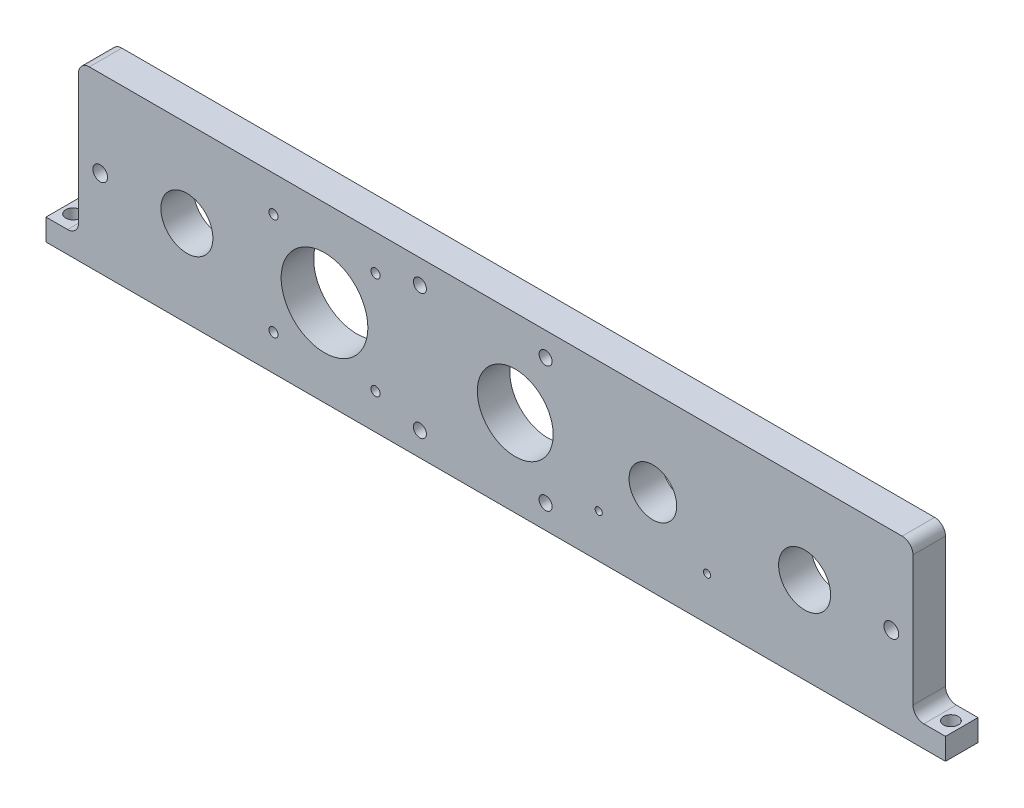
SolidWorks part; units mm, degrees
material "6061 合金"
ref_plane "Front Plane" through (0, 0, 0) normal (0, 0, 1) x (1, 0, 0)
ref_plane "Top Plane" through (0, 0, 0) normal (0, 1, 0) x (1, 0, 0)
ref_plane "Right Plane" through (0, 0, 0) normal (1, 0, 0) x (0, 0, -1)
sketch "Sketch1" plane through (0, 0, 0) normal (0, 0, 1) x (1, 0, 0)
  line L0 (0, 0) -> (0, 85.4446) construction
  line L1 (207.5, 0) -> (-207.5, 0)
  line L2 (-207.5, 0) -> (-207.5, 10)
  line L3 (-207.5, 10) -> (-192.5, 10)
  line L4 (-192.5, 10) -> (-192.5, 70)
  line L5 (-192.5, 70) -> (-207.5, 70)
  line L6 (-207.5, 70) -> (-207.5, 80)
  line L7 (-207.5, 80) -> (207.5, 80)
  line L8 (207.5, 70) -> (207.5, 80)
  line L9 (192.5, 70) -> (207.5, 70)
  line L10 (192.5, 10) -> (192.5, 70)
  line L11 (207.5, 10) -> (192.5, 10)
  line L12 (207.5, 0) -> (207.5, 10)
  point P11 (0, 80)
  dimension "D1" = 80
  dimension "D2" = 10
  dimension "D3" = 10
  dimension "D4" = 15
  dimension "D5" = 415
extrude "Boss-Extrude1" add sketch "Sketch1" along normal mid plane 15
sketch "Sketch2" plane through (0, 0, 7.5) normal (0, 0, 1) x (1, 0, 0)
  line L0 (-192.5, 40) -> (192.5, 40) construction
  line L1 (-192.5, 70) -> (-192.5, 10) construction
  line L2 (192.5, 10) -> (192.5, 70) construction
  circle A0 centre (-142.5, 40) radius 12
  circle A3 centre (9, 40) radius 17.5
  circle A4 centre (72.5, 40) radius 11
  circle A5 centre (-79, 40) radius 20
  circle A6 centre (142.5, 40) radius 12
  circle A7 centre (-182.5, 40) radius 3.4
  circle A8 centre (182.5, 40) radius 3.4
  dimension "D2" = 24
  dimension "D3" = 40
  dimension "D4" = 10
  dimension "D5" = 6.8
  dimension "D6" = 6.8
  dimension "D7" = 63.5
  dimension "D8" = 63.5
  dimension "D9" = 22
  dimension "D10" = 35
  dimension "D11" = 40
  dimension "D12" = 40
  dimension "D13" = 88
  dimension "D14" = 24
  dimension "D15" = 70
  dimension "D16" = 50
  dimension "D17" = 10
extrude "Cut-Extrude1" cut sketch "Sketch2" against normal blind 15
sketch "Sketch3" plane through (0, 0, 7.5) normal (0, 0, 1) x (1, 0, 0)
  line L0 (9, 40) -> (-6, 40) construction
  line L1 (23, 11) -> (-35, 11) construction
  line L2 (23, 11) -> (23, 69) construction
  line L3 (23, 69) -> (-35, 69) construction
  line L4 (-35, 11) -> (-35, 69) construction
  line L5 (23, 11) -> (-35, 69) construction
  line L6 (23, 69) -> (-35, 11) construction
  circle A0 centre (-35, 69) radius 3
  circle A1 centre (23, 69) radius 3
  circle A2 centre (23, 11) radius 3
  circle A3 centre (-35, 11) radius 3
  point P0 (-6, 40)
  dimension "D3" = 6
  dimension "D1" = 58
  dimension "D2" = 15
extrude "Cut-Extrude2" cut sketch "Sketch3" against normal blind 15
sketch "Sketch4" plane through (0, 80, 0) normal (0, 1, 0) x (1, 0, 0)
  line L0 (-207.5, 0) -> (0, 0) construction
  line L1 (-207.5, -7.5) -> (-207.5, 7.5) construction
  line L2 (0, 0) -> (0, 7.5) construction
  line L3 (207.5, 7.5) -> (-207.5, 7.5) construction
  circle A0 centre (-202.5, 0) radius 3.4
  circle A1 centre (202.5, 0) radius 3.4
  dimension "D1" = 6.8
  dimension "D2" = 5
extrude "Cut-Extrude3" cut sketch "Sketch4" against normal through all
fillet "Fillet1" radius 5 4 edges at (-192.5, 10, 0) (-192.5, 70, 0) (192.5, 10, 0) (192.5, 70, 0)
hole_wizard "M4 Tapped Hole1" positions "Sketch6" profile "Sketch7" tap size "M4" standard "GB" end condition through all
sketch "Sketch6" plane through (0, 0, 7.5) normal (0, 0, 1) x (1, 0, 0)
  line L0 (97.5, 20) -> (47.5, 20) construction
  line L2 (72.5, 40) -> (72.5, 20) construction
  point P0 (47.5, 20)
  point P2 (97.5, 20)
  dimension "D1" = 20
  dimension "D2" = 50
sketch "Sketch7" plane through (47.5, 20, 7.5) normal (1, 0, 0) x (0, -1, 0)
  line L0 (0, 0) -> (0, 15)
  line L1 (0, 15) -> (1.65, 15)
  line L2 (1.65, 15) -> (1.65, 0)
  line L5 (1.65, 0) -> (0, 0)
  line L11 (0, -6.35) -> (0, 107.95) construction
  dimension "通孔螺纹孔钻头直径" = 3.3
  dimension "通孔螺纹孔钻头深度" = 15
cosmetic thread "Hole Thread2" parameters "D2"=4
cosmetic thread "Hole Thread7" parameters "D2"=4
hole_wizard "M5 Tapped Hole1" positions "Sketch8" profile "Sketch9" tap size "M5" standard "GB" end condition up to next
sketch "Sketch8" plane through (0, 0, 7.5) normal (0, 0, 1) x (1, 0, 0)
  line L1 (-102.55, 63.55) -> (-55.45, 63.55) construction
  line L2 (-102.55, 63.55) -> (-102.55, 16.45) construction
  line L3 (-102.55, 16.45) -> (-55.45, 16.45) construction
  line L4 (-55.45, 63.55) -> (-55.45, 16.45) construction
  line L5 (-79, 40) -> (-79, 16.45) construction
  line L7 (-55.45, 40) -> (-79, 40) construction
  point P1 (-102.55, 63.55)
  point P2 (-55.45, 16.45)
  point P57 (-102.55, 16.45)
  point P58 (-55.45, 63.55)
  dimension "D1" = 47.1
sketch "Sketch9" plane through (-102.55, 63.55, 7.5) normal (1, 0, 0) x (0, -1, 0)
  line L0 (0, 0) -> (0, 15)
  line L1 (0, 15) -> (2.1, 15)
  line L2 (2.1, 15) -> (2.1, 0)
  line L5 (2.1, 0) -> (0, 0)
  line L11 (0, -6.35) -> (0, 107.95) construction
  dimension "通孔螺纹孔钻头直径" = 4.2
  dimension "通孔螺纹孔钻头深度" = 15
cosmetic thread "Hole Thread3" parameters "D2"=5
cosmetic thread "Hole Thread4" parameters "D2"=5
cosmetic thread "Hole Thread5" parameters "D2"=5
cosmetic thread "Hole Thread6" parameters "D2"=5
sketch "Sketch10" plane through (0, 0, 7.5) normal (0, 0, 1) x (1, 0, 0)
  line L0 (-192.5, 65) -> (-192.5, 15) construction
  line L1 (-192.5, 40) -> (-207.5, 40)
  line L2 (-192.5, 40) -> (-192.5, 80)
  line L3 (-192.5, 80) -> (-207.5, 80)
  line L4 (-207.5, 40) -> (-207.5, 80)
  line L5 (192.5, 15) -> (192.5, 65) construction
  line L6 (192.5, 40) -> (207.5, 40)
  line L7 (192.5, 40) -> (192.5, 80)
  line L8 (192.5, 80) -> (207.5, 80)
  line L9 (207.5, 40) -> (207.5, 80)
extrude "Cut-Extrude4" cut sketch "Sketch10" against normal through all
fillet "Fillet2" radius 5 2 edges at (192.5, 80, 0) (-192.5, 80, 0)
hole_wizard "M6 Tapped Hole1" positions "Sketch11" profile "Sketch12" tap size "M6" standard "GB"
sketch "Sketch11" plane through (0, 0, 0) normal (0, -1, 0) x (-1, 0, 0)
  line L0 (-207.5, 0) -> (-125, 0) construction
  line L1 (-207.5, -7.5) -> (-207.5, 7.5) construction
  line L2 (-125, 0) -> (125, 0) construction
  point P0 (-125, 0)
  point P2 (125, 0)
  dimension "D1" = 250
sketch "Sketch12" plane through (125, 0, 0) normal (1, 0, 0) x (0, 0, -1)
  line L0 (0, 0) -> (0, 16.5022)
  line L1 (0, 16.5022) -> (2.5, 15)
  line L2 (2.5, 15) -> (2.5, 0)
  line L5 (2.5, 0) -> (0, 0)
  line L10 (0, 16.5022) -> (-2.5, 15) construction
  line L11 (0, -6.35) -> (0, 107.95) construction
  dimension "螺纹孔钻头直径" = 5
  dimension "螺纹孔钻头深度" = 15
  dimension "导头角度" = 118
cosmetic thread "Hole Thread8" parameters "D1"=12, "D2"=6
cosmetic thread "Hole Thread9" parameters "D1"=12, "D2"=6
